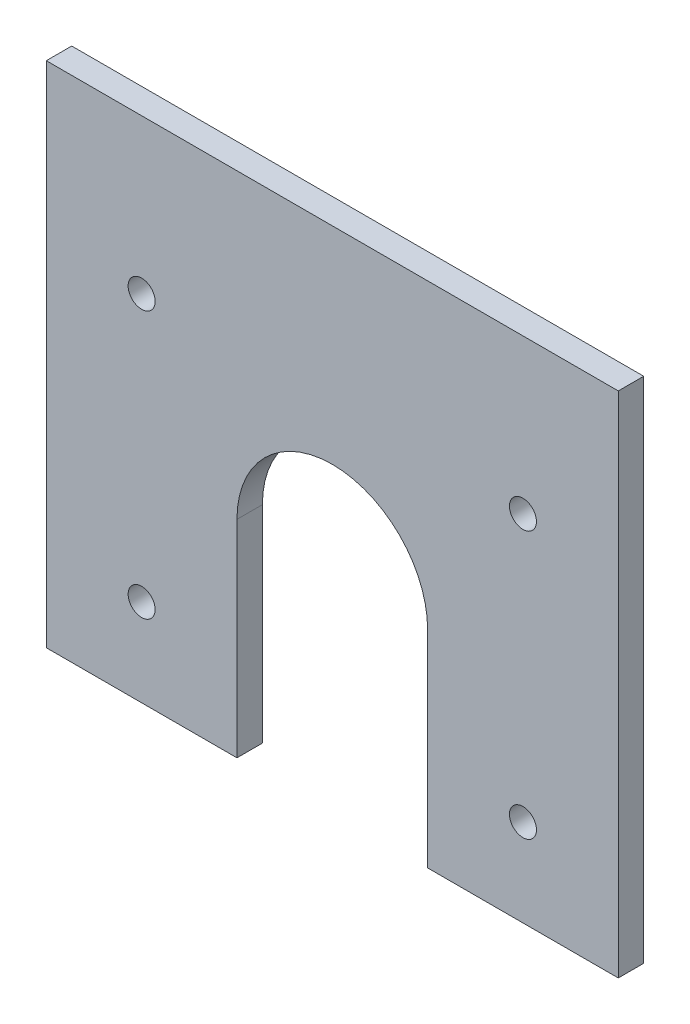
from build123d import *

# Parameters (mm, degrees)
SKETCH1_W            = 360
SKETCH1_H            = 320
EXTRUDE1_DEPTH       = 8
EXTRUDE2_DEPTH       = 16
SKETCH3_R            = 8.5
EXTRUDE3_DEPTH       = 16
LPATTERN1_COUNT      = 2
LPATTERN1_PITCH      = 240
LPATTERN1_COUNT_DIR2 = 2
LPATTERN1_PITCH_DIR2 = 168


with BuildPart() as part:
    # Sketch1 → Extrude1 (new, symmetric)
    with BuildSketch(Plane.XY):
        Rectangle(SKETCH1_W, SKETCH1_H)
    extrude(amount=EXTRUDE1_DEPTH, both=True)

    # Sketch2 → Extrude2 (cut)
    with BuildSketch(Plane.XY.offset(8)):
        with BuildLine():
            Line((-60, -160), (-60, -30))
            ThreePointArc((-60, -30), (0, 30), (60, -30))
            Line((60, -30), (60, -160))
            Line((60, -160), (-60, -160))
        make_face()
    extrude(amount=-EXTRUDE2_DEPTH, mode=Mode.SUBTRACT)

    # Sketch3 → Extrude3 (cut)
    with BuildSketch(Plane.XY.offset(8)):
        with Locations((-120, 63)):
            Circle(SKETCH3_R)
    extrude3 = extrude(amount=-EXTRUDE3_DEPTH, mode=Mode.SUBTRACT)

    # LPattern1: Extrude3 2 × 2
    with Locations(*[(i * LPATTERN1_PITCH, -j * LPATTERN1_PITCH_DIR2, 0) for i in range(LPATTERN1_COUNT) for j in range(LPATTERN1_COUNT_DIR2) if (i, j) != (0, 0)]):
        add(extrude3, mode=Mode.SUBTRACT)


solid = part.part
